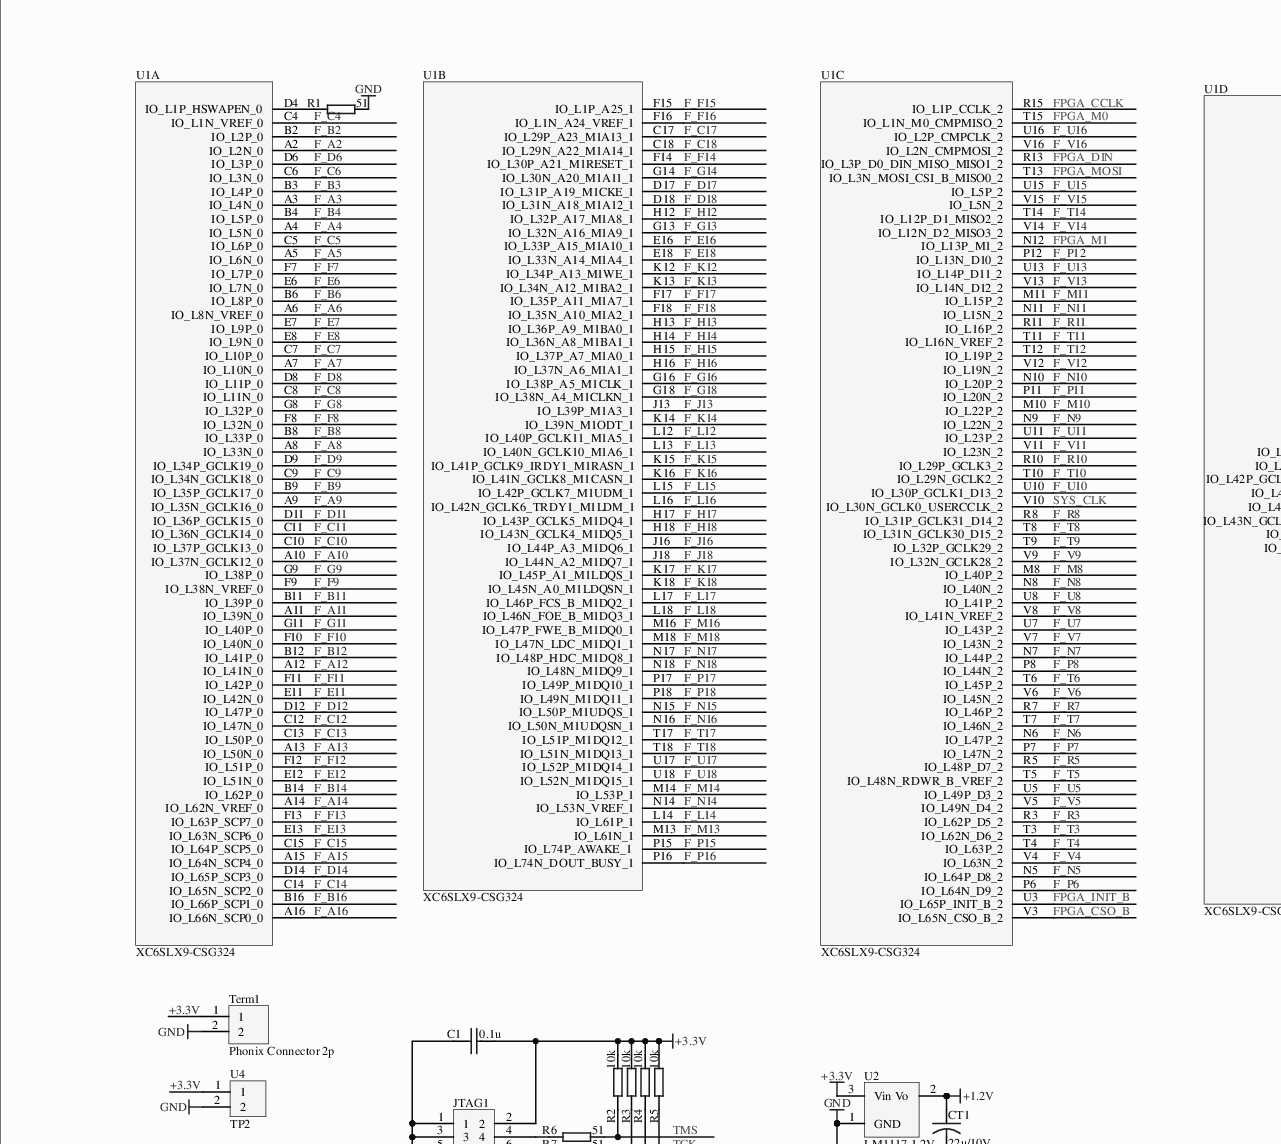
[diagram p0: MISC103828-2.SchDoc, top left]
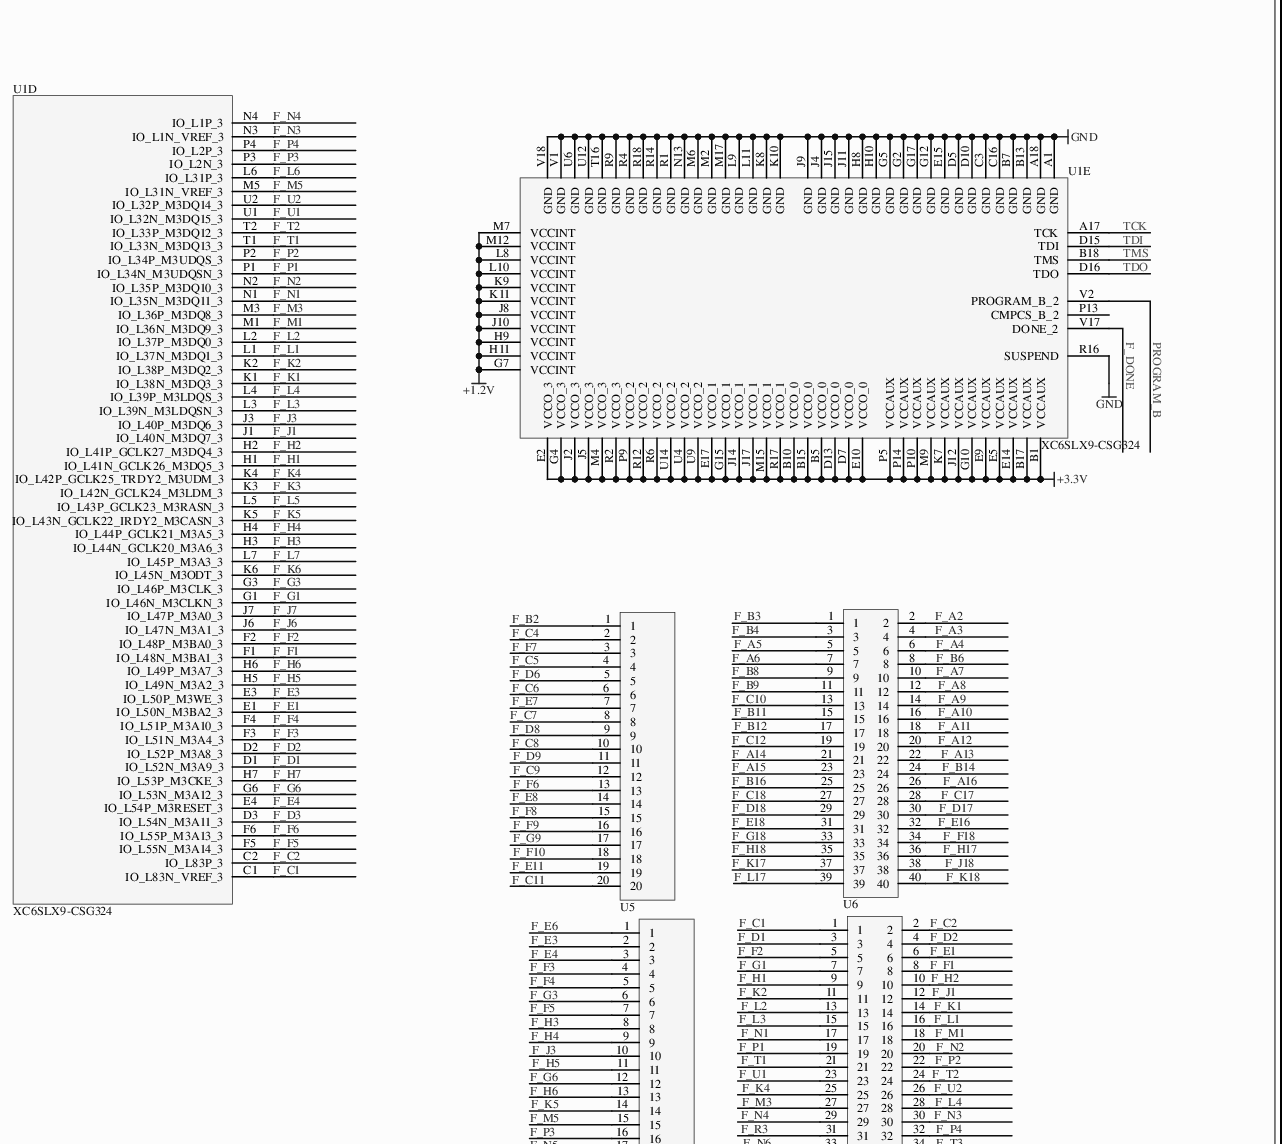
[diagram p1: MISC103828-2.SchDoc, top right]
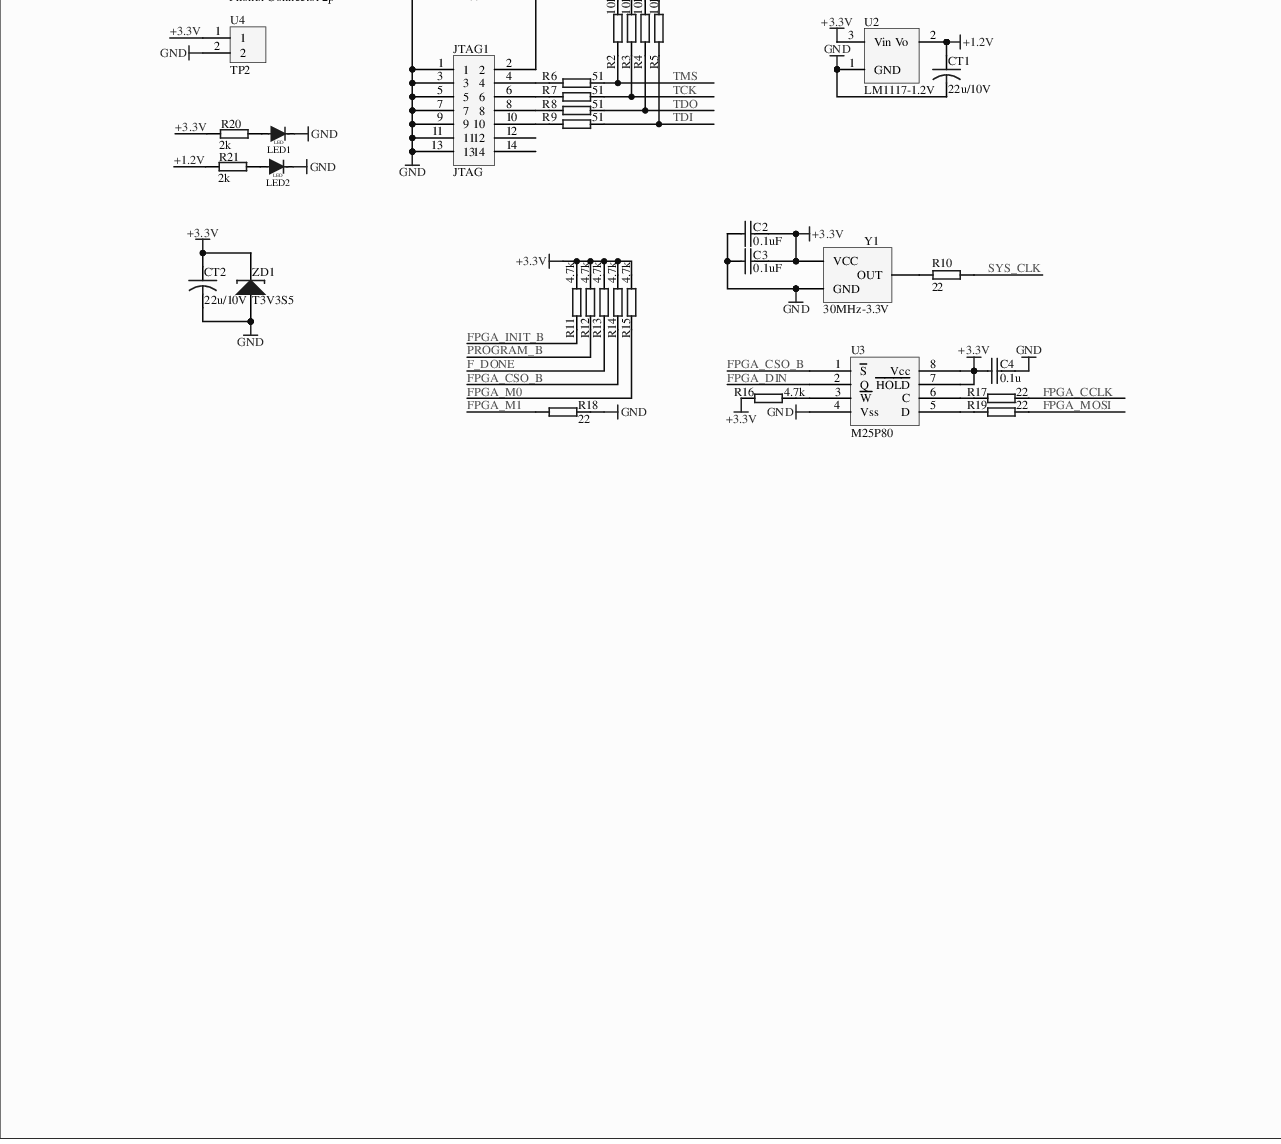
[diagram p2: MISC103828-2.SchDoc, bottom left]
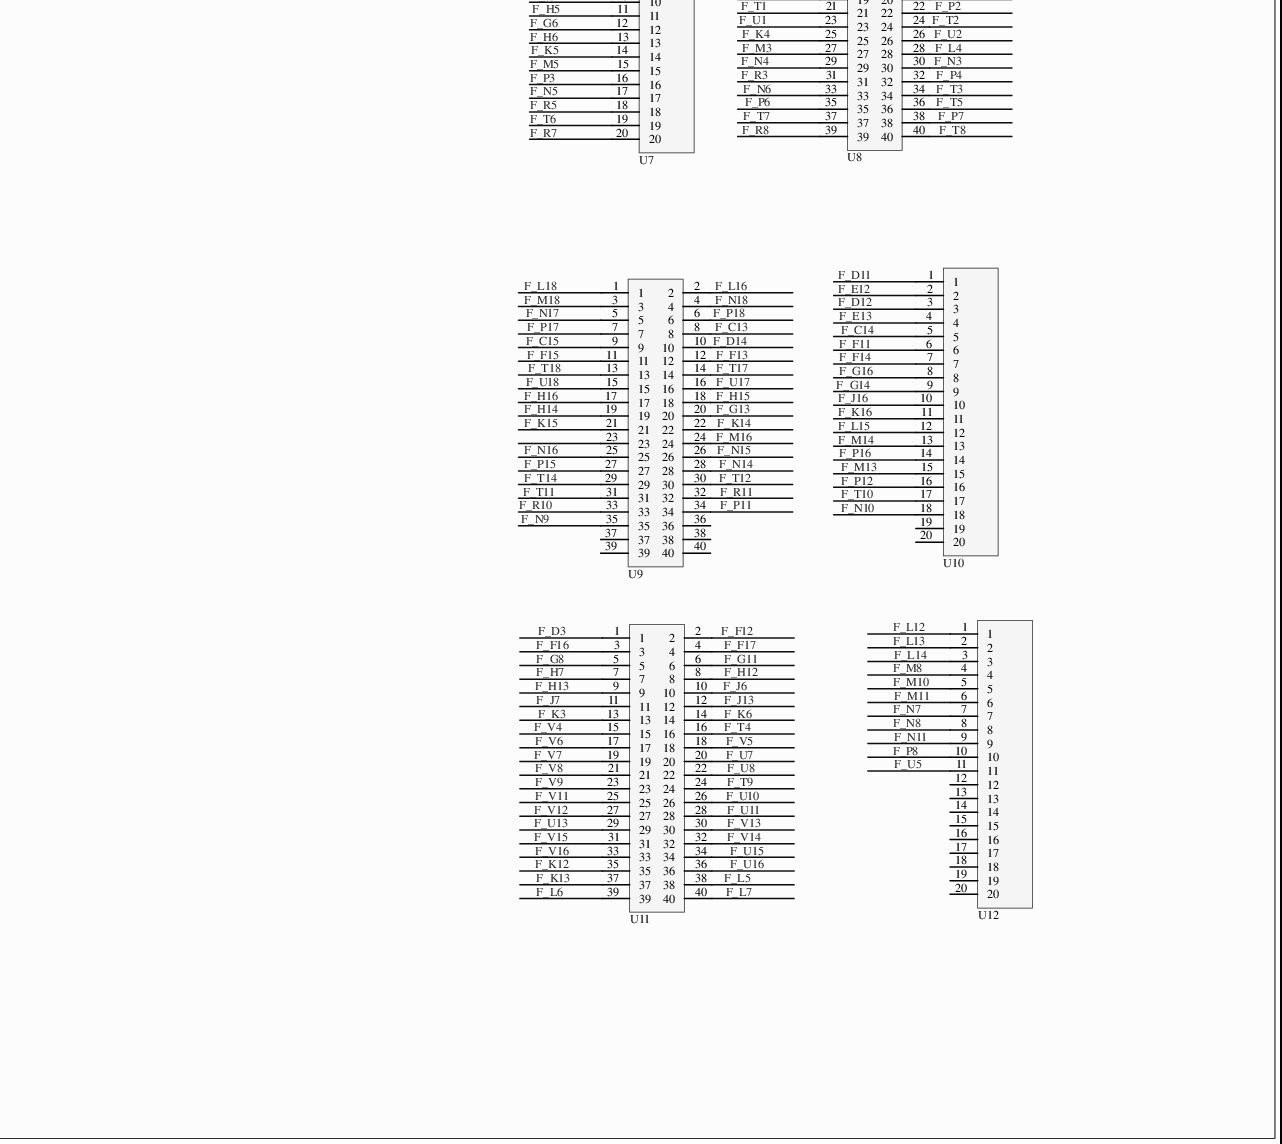
[diagram p3: MISC103828-2.SchDoc, bottom right]
# Altium project MISC103828-6.PrjPcb
1 sheet, 45 parts. Net scope: global (net labels, ports and power ports of the same name join across sheets).
Board file: MISC103828.PcbDoc

## Sheet MISC103828-2.SchDoc
size 457 x 406 mm

### Parts
C1  0.1u  [0603]
C2  0.1uF  [0603]
C3  0.1uF  [0603]
C4  0.1u  [0603]
CT1  22u/10V  [7227]
CT2  22u/10V  [7227]
JTAG1  JTAG  [IDC14S]
LED1  LED  [DIODE_2]  (value not drawn)
LED2  LED  [DIODE_2]  (value not drawn)
R1  51  [0603]
R2  10k  [0603]
R3  10k  [0603]
R4  10k  [0603]
R5  10k  [0603]
R6  51  [0603]
R7  51  [0603]
R8  51  [0603]
R9  51  [0603]
R10  22  [0603]
R11  4.7k  [0603]
R12  4.7k  [0603]
R13  4.7k  [0603]
R14  4.7k  [0603]
R15  4.7k  [0603]
R16  4.7k  [0603]
R17  22  [0603]
R18  22  [0603]
R19  22  [0603]
R20  2k  [0603]
R21  2k  [0603]
Term1  Phonix Connector 2p  [PhonixCon2P]
U1  XC6SLX9-CSG324  [CSG324]  (parts A,B,C,D,E of 5)
U2  LM1117-1.2V  [SOT223]
U3  M25P80  [M25P16_SO-8]
U4  TP2  [TP2]
U5  TP20_2.54mm  [TP20_2.54mm]  (value not drawn)
U6  TP20*2_2.54mm  [TP20*2_2.54mm]  (value not drawn)
U7  TP20_2.54mm  [TP20_2.54mm]  (value not drawn)
U8  TP20*2_2.54mm  [TP20*2_2.54mm]  (value not drawn)
U9  TP20*2_2.54mm  [TP20*2_2.54mm]  (value not drawn)
U10  TP20_2.54mm  [TP20_2.54mm]  (value not drawn)
U11  TP20*2_2.54mm  [TP20*2_2.54mm]  (value not drawn)
U12  TP20_2.54mm  [TP20_2.54mm]  (value not drawn)
Y1  30MHz-3.3V  [OSC-SO4]
ZD1  T3V3S5  [0603]

### Nets
+1.2V: CT1.1 R21.2 U1.G7(VCCINT) U1.H9(VCCINT) U1.H11(VCCINT) U1.J8(VCCINT) U1.J10(VCCINT) U1.K9(VCCINT) U1.K11(VCCINT) U1.L8(VCCINT) U1.L10(VCCINT) U1.M7(VCCINT) U1.M12(VCCINT) U2.2(Vo)
+3.3V: C1.2 C2.2 C3.2 C4.1 CT2.1 JTAG1.2 R2.1 R3.1 R4.1 R5.1 R11.1 R12.1 R13.1 R14.1 R15.1 R16.2 R20.2 Term1.1 U1.B1(VCCAUX) U1.B5(VCCO_0) U1.B10(VCCO_0) U1.B15(VCCO_0) U1.B17(VCCAUX) U1.D7(VCCO_0) U1.D13(VCCO_0) U1.E2(VCCO_3) U1.E5(VCCAUX) U1.E9(VCCAUX) U1.E10(VCCO_0) U1.E14(VCCAUX) U1.E17(VCCO_1) U1.G4(VCCO_3) U1.G10(VCCAUX) U1.G15(VCCO_1) U1.J2(VCCO_3) U1.J5(VCCO_3) U1.J12(VCCAUX) U1.J14(VCCO_1) U1.J17(VCCO_1) U1.K7(VCCAUX) U1.M4(VCCO_3) U1.M9(VCCAUX) U1.M15(VCCO_1) U1.P5(VCCAUX) U1.P9(VCCO_2) U1.P10(VCCAUX) U1.P14(VCCAUX) U1.R2(VCCO_3) U1.R6(VCCO_2) U1.R12(VCCO_2) U1.R17(VCCO_1) U1.U4(VCCO_2) U1.U9(VCCO_2) U1.U14(VCCO_2) U2.3(Vin) U3.7(~{HOLD}) U3.8(Vcc) U4.1 Y1.4(VCC) ZD1.2
GND: C1.1 C2.1 C3.1 C4.2 CT1.2 CT2.2 JTAG1.1 JTAG1.3 JTAG1.5 JTAG1.7 JTAG1.9 JTAG1.11 JTAG1.13 LED1.K LED2.K R1.1 R18.1 Term1.2 U1.A1(GND) U1.A18(GND) U1.B7(GND) U1.B13(GND) U1.C3(GND) U1.C16(GND) U1.D5(GND) U1.D10(GND) U1.E15(GND) U1.G2(GND) U1.G5(GND) U1.G12(GND) U1.G17(GND) U1.H8(GND) U1.H10(GND) U1.J4(GND) U1.J9(GND) U1.J11(GND) U1.J15(GND) U1.K8(GND) U1.K10(GND) U1.L9(GND) U1.L11(GND) U1.M2(GND) U1.M6(GND) U1.M17(GND) U1.N13(GND) U1.R1(GND) U1.R4(GND) U1.R9(GND) U1.R14(GND) U1.R16(SUSPEND) U1.R18(GND) U1.T16(GND) U1.U6(GND) U1.U12(GND) U1.V1(GND) U1.V18(GND) U2.1(GND) U3.4(Vss) U4.2 Y1.2(GND) ZD1.1
F_A2: U1.A2(IO_L2N_0) U6.2
F_A3: U1.A3(IO_L4N_0) U6.4
F_A4: U1.A4(IO_L5N_0) U6.6
F_A5: U1.A5(IO_L6N_0) U6.5
F_A6: U1.A6(IO_L8N_VREF_0) U6.7
F_A7: U1.A7(IO_L10N_0) U6.10
F_A8: U1.A8(IO_L33N_0) U6.12
F_A9: U1.A9(IO_L35N_GCLK16_0) U6.14
F_A10: U1.A10(IO_L37N_GCLK12_0) U6.16
F_A11: U1.A11(IO_L39N_0) U6.18
F_A12: U1.A12(IO_L41N_0) U6.20
F_A13: U1.A13(IO_L50N_0) U6.22
F_A14: U1.A14(IO_L62N_VREF_0) U6.21
F_A15: U1.A15(IO_L64N_SCP4_0) U6.23
F_A16: U1.A16(IO_L66N_SCP0_0) U6.26
F_B2: U1.B2(IO_L2P_0) U5.1
F_B3: U1.B3(IO_L4P_0) U6.1
F_B4: U1.B4(IO_L5P_0) U6.3
F_B6: U1.B6(IO_L8P_0) U6.8
F_B8: U1.B8(IO_L33P_0) U6.9
F_B9: U1.B9(IO_L35P_GCLK17_0) U6.11
F_B11: U1.B11(IO_L39P_0) U6.15
F_B12: U1.B12(IO_L41P_0) U6.17
F_B14: U1.B14(IO_L62P_0) U6.24
F_B16: U1.B16(IO_L66P_SCP1_0) U6.25
F_C1: U1.C1(IO_L83N_VREF_3) U8.1
F_C2: U1.C2(IO_L83P_3) U8.2
F_C4: U1.C4(IO_L1N_VREF_0) U5.2
F_C5: U1.C5(IO_L6P_0) U5.4
F_C6: U1.C6(IO_L3N_0) U5.6
F_C7: U1.C7(IO_L10P_0) U5.8
F_C8: U1.C8(IO_L11N_0) U5.10
F_C9: U1.C9(IO_L34N_GCLK18_0) U5.12
F_C10: U1.C10(IO_L37P_GCLK13_0) U6.13
F_C11: U1.C11(IO_L36N_GCLK14_0) U5.20
F_C12: U1.C12(IO_L47N_0) U6.19
F_C13: U1.C13(IO_L50P_0) U9.8
F_C14: U1.C14(IO_L65N_SCP2_0) U10.5
F_C15: U1.C15(IO_L64P_SCP5_0) U9.9
F_C17: U1.C17(IO_L29P_A23_M1A13_1) U6.28
F_C18: U1.C18(IO_L29N_A22_M1A14_1) U6.27
F_D1: U1.D1(IO_L52N_M3A9_3) U8.3
F_D2: U1.D2(IO_L52P_M3A8_3) U8.4
F_D3: U1.D3(IO_L54N_M3A11_3) U11.1
F_D6: U1.D6(IO_L3P_0) U5.5
F_D8: U1.D8(IO_L11P_0) U5.9
F_D9: U1.D9(IO_L34P_GCLK19_0) U5.11
F_D11: U1.D11(IO_L36P_GCLK15_0) U10.1
F_D12: U1.D12(IO_L47P_0) U10.3
F_D14: U1.D14(IO_L65P_SCP3_0) U9.10
F_D17: U1.D17(IO_L31P_A19_M1CKE_1) U6.30
F_D18: U1.D18(IO_L31N_A18_M1A12_1) U6.29
F_DONE: R13.2 U1.V17(DONE_2)
F_E1: U1.E1(IO_L50N_M3BA2_3) U8.6
F_E3: U1.E3(IO_L50P_M3WE_3) U7.2
F_E4: U1.E4(IO_L54P_M3RESET_3) U7.3
F_E6: U1.E6(IO_L7N_0) U7.1
F_E7: U1.E7(IO_L9P_0) U5.7
F_E8: U1.E8(IO_L9N_0) U5.14
F_E11: U1.E11(IO_L42N_0) U5.19
F_E12: U1.E12(IO_L51N_0) U10.2
F_E13: U1.E13(IO_L63N_SCP6_0) U10.4
F_E16: U1.E16(IO_L33P_A15_M1A10_1) U6.32
F_E18: U1.E18(IO_L33N_A14_M1A4_1) U6.31
F_F1: U1.F1(IO_L48N_M3BA1_3) U8.8
F_F2: U1.F2(IO_L48P_M3BA0_3) U8.5
F_F3: U1.F3(IO_L51N_M3A4_3) U7.4
F_F4: U1.F4(IO_L51P_M3A10_3) U7.5
F_F5: U1.F5(IO_L55N_M3A14_3) U7.7
F_F6: U1.F6(IO_L55P_M3A13_3) U5.13
F_F7: U1.F7(IO_L7P_0) U5.3
F_F8: U1.F8(IO_L32N_0) U5.15
F_F9: U1.F9(IO_L38N_VREF_0) U5.16
F_F10: U1.F10(IO_L40N_0) U5.18
F_F11: U1.F11(IO_L42P_0) U10.6
F_F12: U1.F12(IO_L51P_0) U11.2
F_F13: U1.F13(IO_L63P_SCP7_0) U9.12
F_F14: U1.F14(IO_L30P_A21_M1RESET_1) U10.7
F_F15: U1.F15(IO_L1P_A25_1) U9.11
F_F16: U1.F16(IO_L1N_A24_VREF_1) U11.3
F_F17: U1.F17(IO_L35P_A11_M1A7_1) U11.4
F_F18: U1.F18(IO_L35N_A10_M1A2_1) U6.34
F_G1: U1.G1(IO_L46N_M3CLKN_3) U8.7
F_G3: U1.G3(IO_L46P_M3CLK_3) U7.6
F_G6: U1.G6(IO_L53N_M3A12_3) U7.12
F_G8: U1.G8(IO_L32P_0) U11.5
F_G9: U1.G9(IO_L38P_0) U5.17
F_G11: U1.G11(IO_L40P_0) U11.6
F_G13: U1.G13(IO_L32N_A16_M1A9_1) U9.20
F_G14: U1.G14(IO_L30N_A20_M1A11_1) U10.9
F_G16: U1.G16(IO_L38P_A5_M1CLK_1) U10.8
F_G18: U1.G18(IO_L38N_A4_M1CLKN_1) U6.33
F_H1: U1.H1(IO_L41N_GCLK26_M3DQ5_3) U8.9
F_H2: U1.H2(IO_L41P_GCLK27_M3DQ4_3) U8.10
F_H3: U1.H3(IO_L44N_GCLK20_M3A6_3) U7.8
F_H4: U1.H4(IO_L44P_GCLK21_M3A5_3) U7.9
F_H5: U1.H5(IO_L49N_M3A2_3) U7.11
F_H6: U1.H6(IO_L49P_M3A7_3) U7.13
F_H7: U1.H7(IO_L53P_M3CKE_3) U11.7
F_H12: U1.H12(IO_L32P_A17_M1A8_1) U11.8
F_H13: U1.H13(IO_L36P_A9_M1BA0_1) U11.9
F_H14: U1.H14(IO_L36N_A8_M1BA1_1) U9.19
F_H15: U1.H15(IO_L37P_A7_M1A0_1) U9.18
F_H16: U1.H16(IO_L37N_A6_M1A1_1) U9.17
F_H17: U1.H17(IO_L43P_GCLK5_M1DQ4_1) U6.36
F_H18: U1.H18(IO_L43N_GCLK4_M1DQ5_1) U6.35
F_J1: U1.J1(IO_L40N_M3DQ7_3) U8.12
F_J3: U1.J3(IO_L40P_M3DQ6_3) U7.10
F_J6: U1.J6(IO_L47N_M3A1_3) U11.10
F_J7: U1.J7(IO_L47P_M3A0_3) U11.11
F_J13: U1.J13(IO_L39P_M1A3_1) U11.12
F_J16: U1.J16(IO_L44P_A3_M1DQ6_1) U10.10
F_J18: U1.J18(IO_L44N_A2_M1DQ7_1) U6.38
F_K1: U1.K1(IO_L38N_M3DQ3_3) U8.14
F_K2: U1.K2(IO_L38P_M3DQ2_3) U8.11
F_K3: U1.K3(IO_L42N_GCLK24_M3LDM_3) U11.13
F_K4: U1.K4(IO_L42P_GCLK25_TRDY2_M3UDM_3) U8.25
F_K5: U1.K5(IO_L43N_GCLK22_IRDY2_M3CASN_3) U7.14
F_K6: U1.K6(IO_L45N_M3ODT_3) U11.14
F_K12: U1.K12(IO_L34P_A13_M1WE_1) U11.35
F_K13: U1.K13(IO_L34N_A12_M1BA2_1) U11.37
F_K14: U1.K14(IO_L39N_M1ODT_1) U9.22
F_K15: U1.K15(IO_L41P_GCLK9_IRDY1_M1RASN_1) U9.21
F_K16: U1.K16(IO_L41N_GCLK8_M1CASN_1) U10.11
F_K17: U1.K17(IO_L45P_A1_M1LDQS_1) U6.37
F_K18: U1.K18(IO_L45N_A0_M1LDQSN_1) U6.40
F_L1: U1.L1(IO_L37N_M3DQ1_3) U8.16
F_L2: U1.L2(IO_L37P_M3DQ0_3) U8.13
F_L3: U1.L3(IO_L39N_M3LDQSN_3) U8.15
F_L4: U1.L4(IO_L39P_M3LDQS_3) U8.28
F_L5: U1.L5(IO_L43P_GCLK23_M3RASN_3) U11.38
F_L6: U1.L6(IO_L31P_3) U11.39
F_L7: U1.L7(IO_L45P_M3A3_3) U11.40
F_L12: U1.L12(IO_L40P_GCLK11_M1A5_1) U12.1
F_L13: U1.L13(IO_L40N_GCLK10_M1A6_1) U12.2
F_L14: U1.L14(IO_L61P_1) U12.3
F_L15: U1.L15(IO_L42P_GCLK7_M1UDM_1) U10.12
F_L16: U1.L16(IO_L42N_GCLK6_TRDY1_M1LDM_1) U9.2
F_L17: U1.L17(IO_L46P_FCS_B_M1DQ2_1) U6.39
F_L18: U1.L18(IO_L46N_FOE_B_M1DQ3_1) U9.1
F_M1: U1.M1(IO_L36N_M3DQ9_3) U8.18
F_M3: U1.M3(IO_L36P_M3DQ8_3) U8.27
F_M5: U1.M5(IO_L31N_VREF_3) U7.15
F_M8: U1.M8(IO_L40P_2) U12.4
F_M10: U1.M10(IO_L22P_2) U12.5
F_M11: U1.M11(IO_L15P_2) U12.6
F_M13: U1.M13(IO_L61N_1) U10.15
F_M14: U1.M14(IO_L53P_1) U10.13
F_M16: U1.M16(IO_L47P_FWE_B_M1DQ0_1) U9.24
F_M18: U1.M18(IO_L47N_LDC_M1DQ1_1) U9.3
F_N1: U1.N1(IO_L35N_M3DQ11_3) U8.17
F_N2: U1.N2(IO_L35P_M3DQ10_3) U8.20
F_N3: U1.N3(IO_L1N_VREF_3) U8.30
F_N4: U1.N4(IO_L1P_3) U8.29
F_N5: U1.N5(IO_L64P_D8_2) U7.17
F_N6: U1.N6(IO_L47P_2) U8.33
F_N7: U1.N7(IO_L44P_2) U12.7
F_N8: U1.N8(IO_L40N_2) U12.8
F_N9: U1.N9(IO_L22N_2) U9.35
F_N10: U1.N10(IO_L20P_2) U10.18
F_N11: U1.N11(IO_L15N_2) U12.9
F_N14: U1.N14(IO_L53N_VREF_1) U9.28
F_N15: U1.N15(IO_L50P_M1UDQS_1) U9.26
F_N16: U1.N16(IO_L50N_M1UDQSN_1) U9.25
F_N17: U1.N17(IO_L48P_HDC_M1DQ8_1) U9.5
F_N18: U1.N18(IO_L48N_M1DQ9_1) U9.4
F_P1: U1.P1(IO_L34N_M3UDQSN_3) U8.19
F_P2: U1.P2(IO_L34P_M3UDQS_3) U8.22
F_P3: U1.P3(IO_L2N_3) U7.16
F_P4: U1.P4(IO_L2P_3) U8.32
F_P6: U1.P6(IO_L64N_D9_2) U8.35
F_P7: U1.P7(IO_L47N_2) U8.38
F_P8: U1.P8(IO_L44N_2) U12.10
F_P11: U1.P11(IO_L20N_2) U9.34
F_P12: U1.P12(IO_L13N_D10_2) U10.16
F_P15: U1.P15(IO_L74P_AWAKE_1) U9.27
F_P16: U1.P16(IO_L74N_DOUT_BUSY_1) U10.14
F_P17: U1.P17(IO_L49P_M1DQ10_1) U9.7
F_P18: U1.P18(IO_L49N_M1DQ11_1) U9.6
F_R3: U1.R3(IO_L62P_D5_2) U8.31
F_R5: U1.R5(IO_L48P_D7_2) U7.18
F_R7: U1.R7(IO_L46P_2) U7.20
F_R8: U1.R8(IO_L31P_GCLK31_D14_2) U8.39
F_R10: U1.R10(IO_L29P_GCLK3_2) U9.33
F_R11: U1.R11(IO_L16P_2) U9.32
F_T1: U1.T1(IO_L33N_M3DQ13_3) U8.21
F_T2: U1.T2(IO_L33P_M3DQ12_3) U8.24
F_T3: U1.T3(IO_L62N_D6_2) U8.34
F_T4: U1.T4(IO_L63P_2) U11.16
F_T5: U1.T5(IO_L48N_RDWR_B_VREF_2) U8.36
F_T6: U1.T6(IO_L45P_2) U7.19
F_T7: U1.T7(IO_L46N_2) U8.37
F_T8: U1.T8(IO_L31N_GCLK30_D15_2) U8.40
F_T9: U1.T9(IO_L32P_GCLK29_2) U11.24
F_T10: U1.T10(IO_L29N_GCLK2_2) U10.17
F_T11: U1.T11(IO_L16N_VREF_2) U9.31
F_T12: U1.T12(IO_L19P_2) U9.30
F_T14: U1.T14(IO_L12P_D1_MISO2_2) U9.29
F_T17: U1.T17(IO_L51P_M1DQ12_1) U9.14
F_T18: U1.T18(IO_L51N_M1DQ13_1) U9.13
F_U1: U1.U1(IO_L32N_M3DQ15_3) U8.23
F_U2: U1.U2(IO_L32P_M3DQ14_3) U8.26
F_U5: U1.U5(IO_L49P_D3_2) U12.11
F_U7: U1.U7(IO_L43P_2) U11.20
F_U8: U1.U8(IO_L41P_2) U11.22
F_U10: U1.U10(IO_L30P_GCLK1_D13_2) U11.26
F_U11: U1.U11(IO_L23P_2) U11.28
F_U13: U1.U13(IO_L14P_D11_2) U11.29
F_U15: U1.U15(IO_L5P_2) U11.34
F_U16: U1.U16(IO_L2P_CMPCLK_2) U11.36
F_U17: U1.U17(IO_L52P_M1DQ14_1) U9.16
F_U18: U1.U18(IO_L52N_M1DQ15_1) U9.15
F_V4: U1.V4(IO_L63N_2) U11.15
F_V5: U1.V5(IO_L49N_D4_2) U11.18
F_V6: U1.V6(IO_L45N_2) U11.17
F_V7: U1.V7(IO_L43N_2) U11.19
F_V8: U1.V8(IO_L41N_VREF_2) U11.21
F_V9: U1.V9(IO_L32N_GCLK28_2) U11.23
F_V11: U1.V11(IO_L23N_2) U11.25
F_V12: U1.V12(IO_L19N_2) U11.27
F_V13: U1.V13(IO_L14N_D12_2) U11.30
F_V14: U1.V14(IO_L12N_D2_MISO3_2) U11.32
F_V15: U1.V15(IO_L5N_2) U11.31
F_V16: U1.V16(IO_L2N_CMPMOSI_2) U11.33
FPGA_CCLK: R17.1 U1.R15(IO_L1P_CCLK_2)
FPGA_CSO_B: R14.2 U1.V3(IO_L65N_CSO_B_2) U3.1(~{S})
FPGA_DIN: U1.R13(IO_L3P_D0_DIN_MISO_MISO1_2) U3.2(Q)
FPGA_INIT_B: R11.2 U1.U3(IO_L65P_INIT_B_2)
FPGA_M0: R15.2 U1.T15(IO_L1N_M0_CMPMISO_2)
FPGA_M1: R18.2 U1.N12(IO_L13P_M1_2)
FPGA_MOSI: R19.1 U1.T13(IO_L3N_MOSI_CSI_B_MISO0_2)
PROGRAM_B: R12.2 U1.V2(PROGRAM_B_2)
SYS_CLK: R10.2 U1.V10(IO_L30N_GCLK0_USERCCLK_2)
TCK: R3.2 R7.1 U1.A17(TCK)
TDI: R5.2 R9.1 U1.D15(TDI)
TDO: R4.2 R8.1 U1.D16(TDO)
TMS: R2.2 R6.1 U1.B18(TMS)
NetJTAG1_4: JTAG1.4 R6.2
NetJTAG1_6: JTAG1.6 R7.2
NetJTAG1_8: JTAG1.8 R8.2
NetJTAG1_10: JTAG1.10 R9.2
NetLED1_A: LED1.A R20.1
NetLED2_A: LED2.A R21.1
NetR1_2: R1.2 U1.D4(IO_L1P_HSWAPEN_0)
NetR10_1: R10.1 Y1.3(OUT)
NetR16_1: R16.1 U3.3(~{W})
NetR17_2: R17.2 U3.6(C)
NetR19_2: R19.2 U3.5(D)

Not connected (* = marked no-connect by the designer): JTAG1 12* 14*; U1 P13(CMPCS_B_2)*; U9 23 36 37 38 39 40; U10 19 20; U12 12 13 14 15 16 17 18 19 20

### Library data of the parts
C1 C4 = CAP: Multilayer ceramic capacitor
C2 C3 = CAP: Capacitor
CT1 CT2 = CAPACITOR
JTAG1 = IDC14
R1-R21 = RES2
U1 = XC6SLX25-CSG324
U2 = 7810
Y1 = OSCILLATOR
ZD1 = D Tunnel2: Tunnel Diode - Dependent Source Model